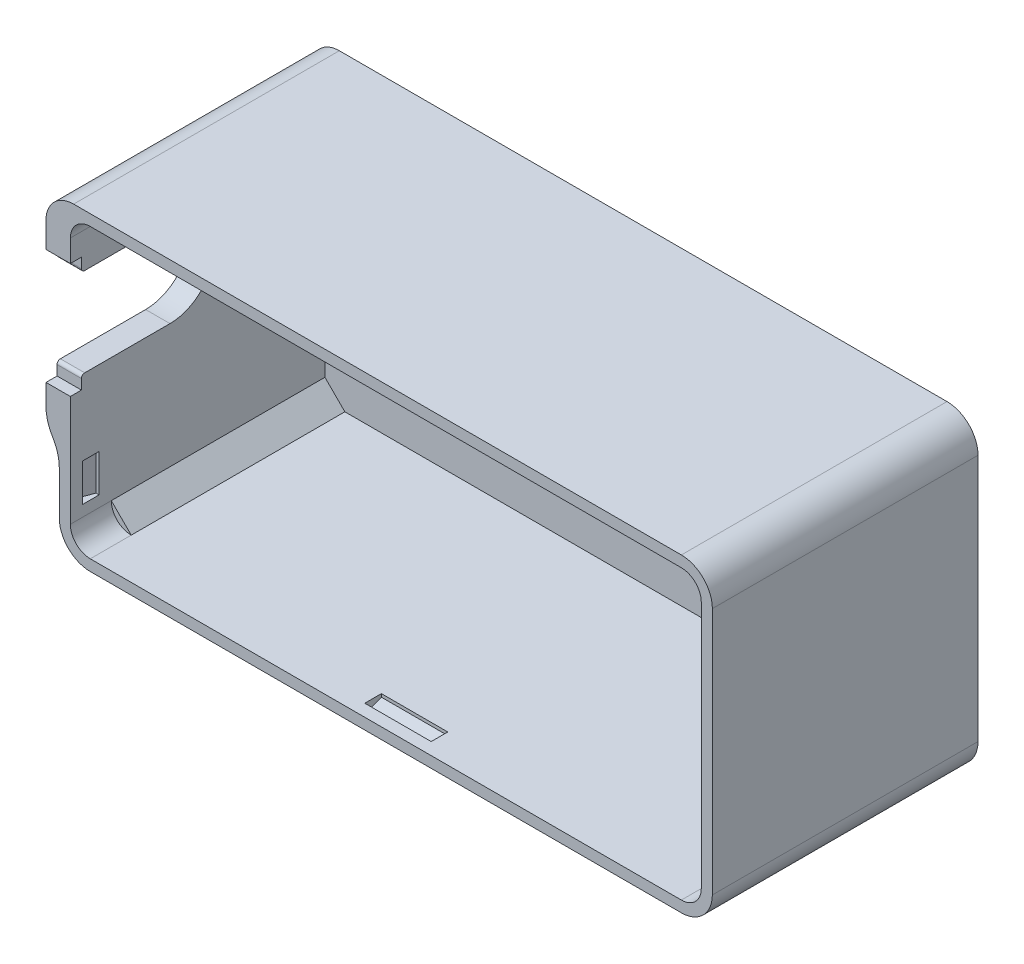
from build123d import *

# Parameters (mm, degrees)
EXTRUDE_1_DEPTH       = 23
EXTRUDE_START         = 1
EXTRUDE_2_DEPTH       = 1
CUT_EXTRUDE_1_DEPTH   = 20
SKETCH_5_W            = 3.764983414
SKETCH_5_H            = 10.4
CUT_EXTRUDE_3_DEPTH   = 10
CUT_EXTRUDE_START     = 6.8
CUT_EXTRUDE_4_DEPTH   = 3.4
MIRROR_START          = 6.8
MIRROR_2_COPY_1_DEPTH = 3.4
FILLET_2_R            = 0.3
EXTRUDE_3_DEPTH       = 19.3
EXTRUDE_START_2       = -24
EXTRUDE_4_DEPTH       = 24
CUT_EXTRUDE_START_2   = -10
CUT_EXTRUDE_5_DEPTH   = 10
EXTRUDE_START_3       = -2.2
EXTRUDE_5_DEPTH       = 2.2
CUT_EXTRUDE_6_DEPTH   = 5
CUT_EXTRUDE_7_DEPTH   = 3


with BuildPart() as part:
    # 草图1 → 凸台-拉伸1 (new body)
    with BuildSketch(Plane.XY):
        with BuildLine():
            Line((-26.7, 14), (26.7, 14))
            ThreePointArc((26.7, 14), (28.679898987, 13.179898987), (29.5, 11.2))
            Line((29.5, 11.2), (29.5, -11.2))
            ThreePointArc((29.5, -11.2), (28.679898987, -13.179898987), (26.7, -14))
            Line((26.7, -14), (-26.7, -14))
            ThreePointArc((-26.7, -14), (-28.679898987, -13.179898987), (-29.5, -11.2))
            Line((-29.5, -11.2), (-29.5, 11.2))
            ThreePointArc((-29.5, 11.2), (-28.679898987, 13.179898987), (-26.7, 14))
        make_face()
        with BuildLine():
            Line((-26.7, 13), (26.7, 13))
            ThreePointArc((26.7, 13), (27.972792206, 12.472792206), (28.5, 11.2))
            Line((28.5, 11.2), (28.5, -11.2))
            ThreePointArc((28.5, -11.2), (27.972792206, -12.472792206), (26.7, -13))
            Line((26.7, -13), (-26.7, -13))
            ThreePointArc((-26.7, -13), (-27.972792206, -12.472792206), (-28.5, -11.2))
            Line((-28.5, -11.2), (-28.5, 11.2))
            ThreePointArc((-28.5, 11.2), (-27.972792206, 12.472792206), (-26.7, 13))
        make_face(mode=Mode.SUBTRACT)
    extrude(amount=EXTRUDE_1_DEPTH)

    # 草图2 → 凸台-拉伸2 (add)
    with BuildSketch(Plane(origin=(0, 0, 0), x_dir=(-1, 0, 0), z_dir=(0, 0, -1)).offset(EXTRUDE_START)):
        with BuildLine():
            Line((26.7, 14), (-26.7, 14))
            ThreePointArc((-26.7, 14), (-28.679898987, 13.179898987), (-29.5, 11.2))
            Line((-29.5, 11.2), (-29.5, -11.2))
            ThreePointArc((-29.5, -11.2), (-28.679898987, -13.179898987), (-26.7, -14))
            Line((-26.7, -14), (26.7, -14))
            ThreePointArc((26.7, -14), (28.679898987, -13.179898987), (29.5, -11.2))
            Line((29.5, -11.2), (29.5, 11.2))
            ThreePointArc((29.5, 11.2), (28.679898987, 13.179898987), (26.7, 14))
        make_face()
    extrude(amount=-EXTRUDE_2_DEPTH)

    # 草图3 → 切除-拉伸1 (cut)
    with BuildSketch(Plane.ZY.offset(29.5)):
        with BuildLine():
            Line((14, 8), (25.240812318, 8))
            Line((25.240812318, 8), (25.240812318, 0))
            Line((25.240812318, 0), (14, 0))
            ThreePointArc((14, 0), (10, 4), (14, 8))
        make_face()
    extrude(amount=-CUT_EXTRUDE_1_DEPTH, mode=Mode.SUBTRACT)

    # 草图5 → 切除-拉伸3 (cut)
    with BuildSketch(Plane.ZY.offset(29.5)):
        with Locations((23.882491707, 4)):
            Rectangle(SKETCH_5_W, SKETCH_5_H)
    extrude(amount=-CUT_EXTRUDE_3_DEPTH, mode=Mode.SUBTRACT)

    # 草图6 → 切除-拉伸4 (cut)
    with BuildSketch(Plane(origin=(0, 0, 0), x_dir=(1, 0, 0), z_dir=(0, 1, 0)).offset(CUT_EXTRUDE_START)):
        Polygon((-28.5, -21.9), (-29.2, -21.9), (-29.2, -21.55), (-28.781434231, -20.4), (-28.5, -20.4), align=None)
    cut_extrude_4 = extrude(amount=CUT_EXTRUDE_4_DEPTH, mode=Mode.SUBTRACT)

    # 镜向1: 切除-拉伸4 across plane
    add(cut_extrude_4.mirror(Plane.ZX), mode=Mode.SUBTRACT)

    # 镜向2: 切除-拉伸4 across plane
    add(cut_extrude_4.mirror(Plane(origin=(0, 0, 0), x_dir=(0, 0, 1), z_dir=(1, 0, 0))), mode=Mode.SUBTRACT)

    # 镜向2 copy 1 sketch → 镜向2 copy 1 (cut)
    with BuildSketch(Plane(origin=(0, 0, 0), x_dir=(-1, 0, 0), z_dir=(0, -1, 0)).offset(MIRROR_START)):
        Polygon((-28.5, -21.9), (-29.2, -21.9), (-29.2, -21.55), (-28.781434231, -20.4), (-28.5, -20.4), align=None)
    extrude(amount=MIRROR_2_COPY_1_DEPTH, mode=Mode.SUBTRACT)

    # 圆角2
    fillet_2_edges = [part.edges().sort_by_distance(p)[0] for p in [
        (-29, 0, 22),
        (-29, 8, 22),
    ]]
    fillet(fillet_2_edges, radius=FILLET_2_R)

    # 草图9 → 凸台-拉伸3 (add)
    with BuildSketch(Plane.XY):
        with BuildLine():
            Line((-28.5, 11.2), (-26.7, 13))
            ThreePointArc((-26.7, 13), (-27.972792206, 12.472792206), (-28.5, 11.2))
        make_face()
        with BuildLine():
            Line((28.5, 11.2), (26.7, 13))
            ThreePointArc((26.7, 13), (27.972792206, 12.472792206), (28.5, 11.2))
        make_face()
        with BuildLine():
            Line((28.5, -11.2), (26.7, -13))
            ThreePointArc((26.7, -13), (27.972792206, -12.472792206), (28.5, -11.2))
        make_face()
        with BuildLine():
            Line((-28.5, -11.2), (-26.7, -13))
            ThreePointArc((-26.7, -13), (-27.972792206, -12.472792206), (-28.5, -11.2))
        make_face()
    extrude(amount=EXTRUDE_3_DEPTH)

    # 草图11 → 凸台-拉伸4 (add)
    with BuildSketch(Plane.XY.offset(23).offset(EXTRUDE_START_2)):
        with BuildLine():
            Line((-30.7, -3.068055681), (-30.7, 11.5))
            ThreePointArc((-30.7, 11.5), (-29.967766953, 13.267766953), (-28.2, 14))
            Line((-28.2, 14), (-26.7, 14))
            ThreePointArc((-26.7, 14), (-28.679898987, 13.179898987), (-29.5, 11.2))
            Line((-29.5, 11.2), (-29.5, -7.286930049))
            ThreePointArc((-29.5, -7.286930049), (-29.639971651, -6.238034848), (-30.050090571, -5.262547444))
            Line((-30.050090571, -5.262547444), (-30.149909429, -5.092438287))
            ThreePointArc((-30.149909429, -5.092438287), (-30.560028349, -4.116950882), (-30.7, -3.068055681))
        make_face()
    extrude(amount=EXTRUDE_4_DEPTH)

    # 草图12 → 切除-拉伸5 (cut)
    with BuildSketch(Plane(origin=(-29.5, 0, 0), x_dir=(0, 0, -1), z_dir=(1, 0, 0)).offset(CUT_EXTRUDE_START_2)):
        with BuildLine():
            Line((-23, 9.2), (-23, -1.2))
            Line((-23, -1.2), (-22, -1.2))
            Line((-22, -1.2), (-22, -0.3))
            ThreePointArc((-22, -0.3), (-21.912132034, -0.087867966), (-21.7, 0))
            Line((-21.7, 0), (-14, 0))
            ThreePointArc((-14, 0), (-10, 4), (-14, 8))
            Line((-14, 8), (-21.7, 8))
            ThreePointArc((-21.7, 8), (-21.912132034, 8.087867966), (-22, 8.3))
            Line((-22, 8.3), (-22, 9.2))
            Line((-22, 9.2), (-23, 9.2))
        make_face()
    extrude(amount=CUT_EXTRUDE_5_DEPTH, mode=Mode.SUBTRACT)

    # 草图13 → 凸台-拉伸5 (add)
    with BuildSketch(Plane.XZ.offset(-8).offset(EXTRUDE_START_3)):
        Polygon((-28.5, 20.4), (-28.5, 21.9), (-29.2, 21.9), (-29.2, 21.55), (-28.781434231, 20.4), align=None)
    extrude(amount=EXTRUDE_5_DEPTH)

    # 草图14 → 切除-拉伸6 (cut)
    with BuildSketch(Plane.ZY.offset(29.2)):
        with BuildLine():
            Line((21.7, 8), (22.114153774, 8))
            Line((22.114153774, 8), (22, 8.3))
            ThreePointArc((22, 8.3), (21.912132034, 8.087867966), (21.7, 8))
        make_face()
    extrude(amount=-CUT_EXTRUDE_6_DEPTH, mode=Mode.SUBTRACT)

    # 草图10 → 切除-拉伸7 (cut, symmetric)
    with BuildSketch(Plane.ZY):
        Polygon((21.9, -13.7), (21.9, -13), (20.4, -13), (20.4, -13.281434231), (21.55, -13.7), align=None)
    cut_extrude_7 = extrude(amount=CUT_EXTRUDE_7_DEPTH, both=True, mode=Mode.SUBTRACT)

    # 镜向3: 切除-拉伸7 across plane
    add(cut_extrude_7.mirror(Plane.ZX), mode=Mode.SUBTRACT)


solid = part.part
